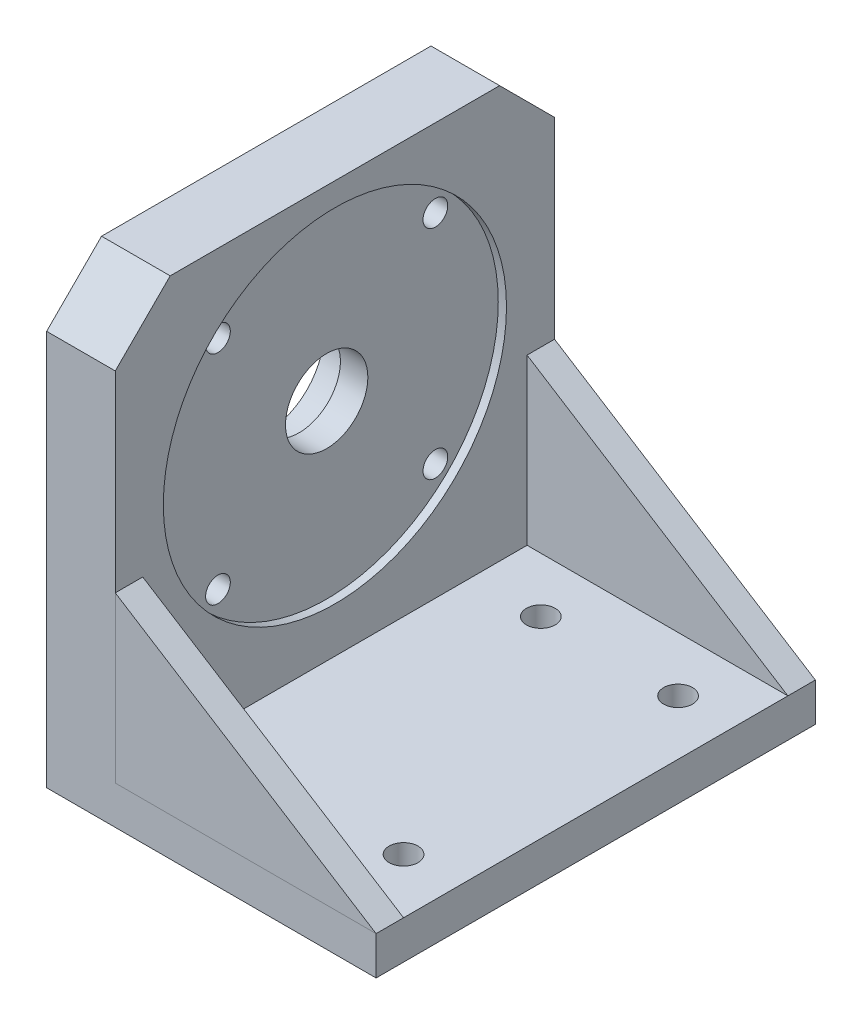
SolidWorks part; units mm, degrees
ref_plane "前视基准面" through (0, 0, 0) normal (0, 0, 1) x (1, 0, 0)
ref_plane "上视基准面" through (0, 0, 0) normal (0, 1, 0) x (1, 0, 0)
ref_plane "右视基准面" through (0, 0, 0) normal (1, 0, 0) x (0, 0, -1)
sketch "草图1" plane through (0, 0, 0) normal (0, 1, 0) x (1, 0, 0)
  line L1 (-60, 80) -> (60, 80)
  line L2 (-60, 80) -> (-60, -80)
  line L3 (-60, -80) -> (60, -80)
  line L4 (60, 80) -> (60, -80)
  line L5 (-60, 80) -> (60, -80) construction
  line L6 (-60, -80) -> (60, 80) construction
  point P0 (0, 0)
  dimension "D1" = 120
  dimension "D2" = 160
extrude "凸台-拉伸1" add sketch "草图1" along normal blind 14
sketch "草图2" plane through (0, 14, 0) normal (0, 1, 0) x (1, 0, 0)
  line L0 (-60, -80) -> (60, -80) construction
  line L1 (-60, 80) -> (-35, 80)
  line L2 (-60, 80) -> (-60, -80)
  line L3 (-60, -80) -> (-35, -80)
  line L4 (-35, 80) -> (-35, -80)
  dimension "D1" = 25
extrude "凸台-拉伸2" add sketch "草图2" along normal blind 150
sketch "草图3" plane through (0, 0, 80) normal (0, 0, 1) x (1, 0, 0)
  line L0 (-35, 74) -> (60, 14)
  line L1 (-35, 164) -> (-35, 14) construction
  line L2 (-35, 14) -> (60, 14) construction
  line L3 (-35, 74) -> (-35, 14)
  line L4 (-35, 14) -> (60, 14)
  dimension "D1" = 60
extrude "凸台-拉伸3" add sketch "草图3" against normal blind 10 separate body
sketch "草图4" plane through (0, 0, -80) normal (0, 0, -1) x (-1, 0, 0)
  line L3 (35, 14) -> (35, 74)
  line L4 (35, 74) -> (-60, 14)
  line L5 (35, 14) -> (35, 74)
  line L7 (35, 74) -> (-60, 14)
  line L9 (-60, 14) -> (35, 14)
  line L10 (-60, 14) -> (35, 14)
  dimension "D1" = 0
extrude "凸台-拉伸4" add sketch "草图4" against normal blind 10 separate body
sketch "草图5" plane through (-60, 0, 0) normal (-1, 0, 0) x (0, 0, 1)
  line L0 (-80, 0) -> (80, 0) construction
  circle A0 centre (0, 93) radius 21
  dimension "D1" = 93
  dimension "D2" = 42
extrude "切除-拉伸1" cut sketch "草图5" against normal blind 12
sketch "草图6" plane through (-48, 0, 0) normal (-1, 0, 0) x (0, 0, 1)
  circle A0 centre (0, 93) radius 15
  dimension "D1" = 30
extrude "切除-拉伸2" cut sketch "草图6" against normal through all
sketch "草图7" plane through (-35, 0, 0) normal (1, 0, 0) x (0, 0, -1)
  circle A0 centre (0, 93) radius 62.5
  dimension "D1" = 125
extrude "切除-拉伸3" cut sketch "草图7" against normal blind 3
hole_wizard "Ø10.5 (10.5) 直径孔1" positions "草图8" profile "草图9" hole size "Ø10.5" standard "GB"
sketch "草图8" plane through (0, 14, 0) normal (0, 1, 0) x (1, 0, 0)
  line L0 (0, 0) -> (45.5582, 0) construction
  line L2 (60, -80) -> (60, 80) construction
  point P0 (40, 50)
  point P2 (40, -50)
  dimension "D1" = 100
  dimension "D2" = 20
sketch "草图9" plane through (40, 14, -50) normal (1, 0, 0) x (0, 0, 1)
  line L0 (0, 0) -> (0, 18.1545)
  line L1 (0, 18.1545) -> (5.25, 15)
  line L2 (5.25, 15) -> (5.25, 0)
  line L5 (5.25, 0) -> (0, 0)
  line L10 (0, 18.1545) -> (-5.25, 15) construction
  line L11 (0, -6.35) -> (0, 107.95) construction
  dimension "孔直径" = 10.5
  dimension "孔深度" = 15
  dimension "导头角度" = 118
pattern_linear "阵列(线性)1" count 2 spacing 50 along (-1, 0, 0) of "Ø10.5 (10.5) 直径孔1"
chamfer "倒角1" distance 20 angle 45 2 edges at (-47.5, 164, 80) (-47.5, 164, -80)
hole_wizard "打孔尺寸(%根据)内六角圆柱头螺钉的类型1" positions "草图10" profile "草图11" counterbore size "M8" standard "GB" end condition through all
sketch "草图10" plane through (-60, 0, 0) normal (-1, 0, 0) x (0, 0, 1)
  line L0 (0, 93) -> (-39.598, 132.598) construction
  line L2 (0, 93) -> (0, 141.5405) construction
  point P0 (-39.598, 132.598)
  dimension "D1" = 45
  dimension "D2" = 56
sketch "草图11" plane through (-60, 132.598, -39.598) normal (0, 1, 0) x (0, 0, 1)
  line L0 (0, 0) -> (0, 120)
  line L1 (0, 120) -> (4.5, 120)
  line L3 (4.5, 120) -> (4.5, 9)
  line L4 (4.5, 9) -> (7.5, 9)
  line L5 (7.5, 9) -> (7.5, 0)
  line L7 (7.5, 0) -> (0, 0)
  line L11 (0, -6.35) -> (0, 107.95) construction
  dimension "通孔孔直径" = 9
  dimension "通孔孔深度" = 120
  dimension "柱形沉头孔直径" = 15
  dimension "柱形沉头孔深度" = 9
pattern_circular "阵列(圆周)1" count 4 over 360 about axis through (0, 93, 0) along (1, 0, 0) of "打孔尺寸(%根据)内六角圆柱头螺钉的类型1"
